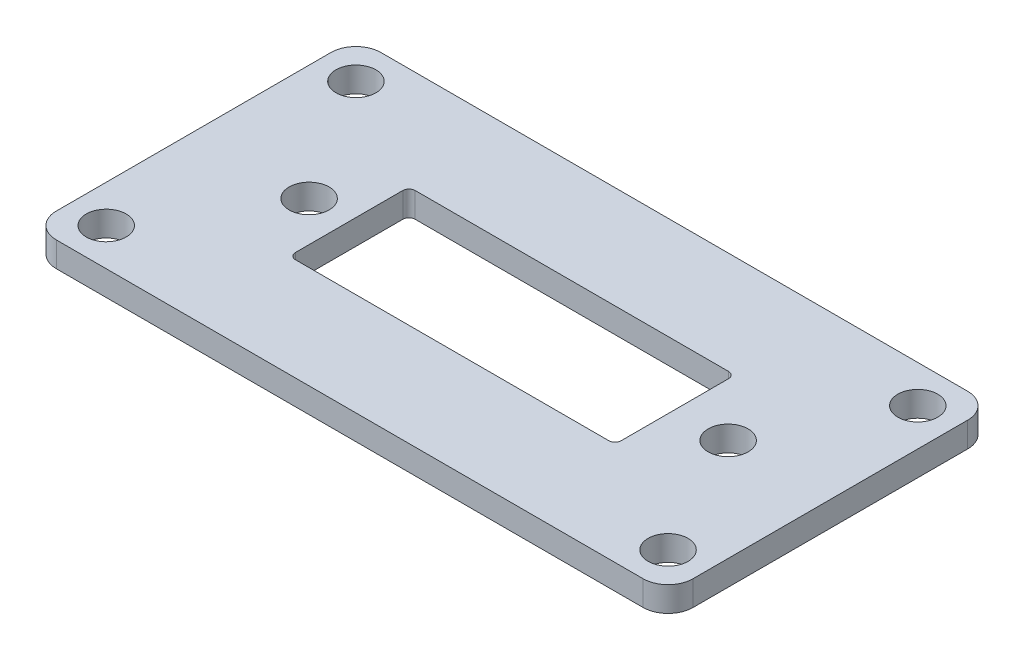
SolidWorks part; units mm, degrees
ref_plane "Front Plane" through (0, 0, 0) normal (0, 0, 1) x (1, 0, 0)
ref_plane "Top Plane" through (0, 0, 0) normal (0, 1, 0) x (1, 0, 0)
ref_plane "Right Plane" through (0, 0, 0) normal (1, 0, 0) x (0, 0, -1)
sketch "Sketch1" plane through (0, 0, 0) normal (0, 1, 0) x (1, 0, 0)
  line L1 (-22.5, -10) -> (22.5, -10) construction
  line L2 (-22.5, -10) -> (-22.5, 10) construction
  line L3 (-22.5, 10) -> (22.5, 10) construction
  line L4 (22.5, -10) -> (22.5, 10) construction
  line L5 (-22.5, -10) -> (22.5, 10) construction
  line L6 (-22.5, 10) -> (22.5, -10) construction
  line L7 (-23.5, -13) -> (23.5, -13)
  line L8 (-25.5, -11) -> (-25.5, 11)
  line L9 (-23.5, 13) -> (23.5, 13)
  line L10 (25.5, -11) -> (25.5, 11)
  line L11 (-25.5, -13) -> (25.5, 13) construction
  line L12 (-25.5, 13) -> (25.5, -13) construction
  circle A0 centre (-22.5, 10) radius 1.6
  circle A1 centre (22.5, 10) radius 1.6
  circle A2 centre (22.5, -10) radius 1.6
  circle A3 centre (-22.5, -10) radius 1.6
  arc A4 (23.5, 13) -> (25.5, 11) centre (23.5, 11) cw
  arc A5 (23.5, -13) -> (25.5, -11) centre (23.5, -11) ccw
  arc A6 (-23.5, -13) -> (-25.5, -11) centre (-23.5, -11) cw
  arc A7 (-25.5, 11) -> (-23.5, 13) centre (-23.5, 11) cw
  point P0 (0, 0)
  point P6 (0, 0)
  dimension "D3" = 3.2
  dimension "D4" = 3.2
  dimension "D5" = 3.2
  dimension "D6" = 3.2
  dimension "D9" = 2
  dimension "D1" = 45
  dimension "D2" = 20
  dimension "D7" = 51
  dimension "D8" = 26
extrude "Boss-Extrude1" add sketch "Sketch1" along normal blind 2
sketch "Sketch2" plane through (0, 0, 0) normal (0, -1, 0) x (1, 0, 0)
  line L0 (-19, 7.5) -> (19, 7.5) construction
  line L1 (-20, -7.5) -> (20, -7.5) construction
  line L2 (-20, -7.5) -> (-20, 7.5) construction
  line L3 (-20, 7.5) -> (20, 7.5) construction
  line L4 (20, -7.5) -> (20, 7.5) construction
  line L5 (-20, -7.5) -> (20, 7.5) construction
  line L6 (-20, 7.5) -> (20, -7.5) construction
  line L9 (-13.05, -4.8) -> (13.05, -4.8)
  line L10 (-13.05, -4.8) -> (-13.05, 4.8)
  line L11 (-13.05, 4.8) -> (13.05, 4.8)
  line L12 (13.05, -4.8) -> (13.05, 4.8)
  line L13 (-13.05, -4.8) -> (13.05, 4.8) construction
  line L14 (-13.05, 4.8) -> (13.05, -4.8) construction
  circle A0 centre (-16.25, 0) radius 1.6
  circle A1 centre (17.3113, 0) radius 1.6
  point P0 (0, 0)
  point P8 (0, 0)
  dimension "D4" = 16.25
  dimension "D5" = 3.2
  dimension "D6" = 3.2
  dimension "D1" = 40
  dimension "D2" = 26.1
  dimension "D3" = 9.6
extrude "Cut-Extrude1" cut sketch "Sketch2" against normal blind 2
fillet "Fillet1" radius 0.5 4 edges at (-13.05, 1, 4.8) (13.05, 1, 4.8) (13.05, 1, -4.8) (-13.05, 1, -4.8)
